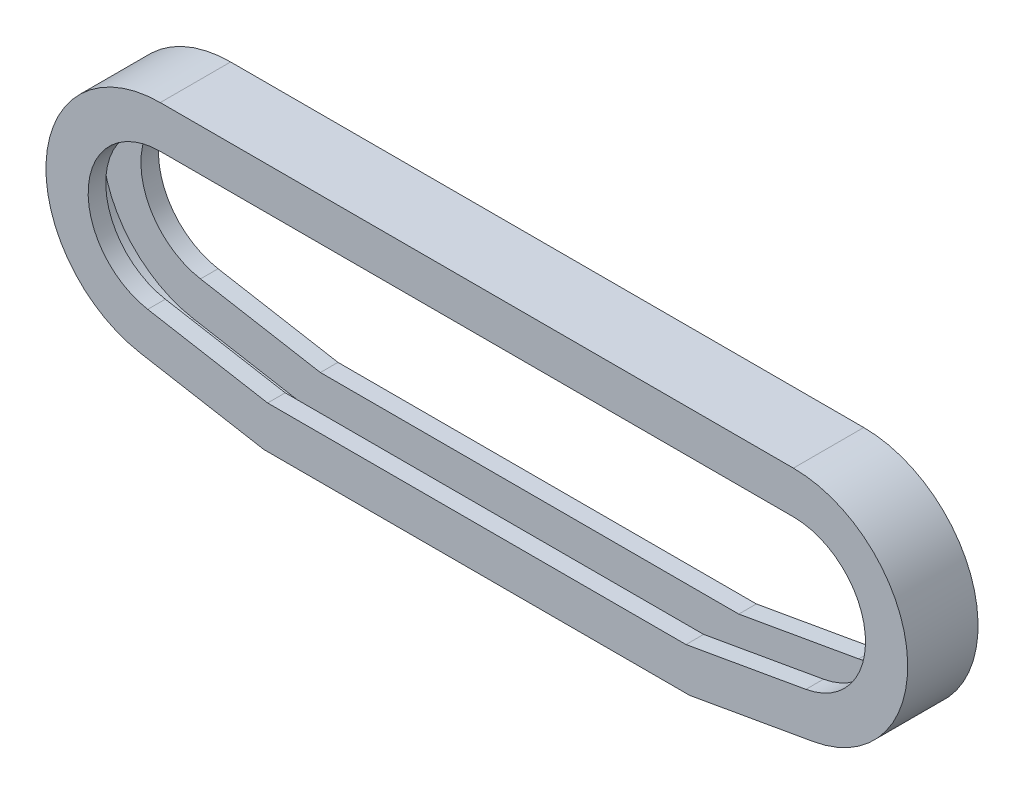
SolidWorks part; units mm, degrees
ref_plane "Front Plane" through (0, 0, 0) normal (0, 0, 1) x (1, 0, 0)
ref_plane "Top Plane" through (0, 0, 0) normal (0, 1, 0) x (1, 0, 0)
ref_plane "Right Plane" through (0, 0, 0) normal (1, 0, 0) x (0, 0, -1)
sketch "Sketch2" plane through (0, 0, 0) normal (0, 0, 1) x (1, 0, 0)
  line L0 (90, 0) -> (-90, 0) construction
  line L1 (0, 0) -> (0, -32.1986) construction
  line L2 (-60, -32.1986) -> (-94.6017, -26.0974) construction
  line L3 (60, -32.1986) -> (94.6017, -26.0974) construction
  line L4 (-90, 26.5) -> (90, 26.5) construction
  line L5 (-60, -32.1986) -> (60, -32.1986) construction
  line L6 (-90, 0) -> (-94.6017, -26.0974) construction
  line L7 (-90, 32.5) -> (90, 32.5)
  line L8 (60.5249, -38.1986) -> (95.6436, -32.0063)
  line L9 (-60.5249, -38.1986) -> (60.5249, -38.1986)
  line L10 (-60.5249, -38.1986) -> (-95.6436, -32.0063)
  line L11 (-90, 20.5) -> (90, 20.5)
  line L12 (59.4751, -26.1986) -> (93.5598, -20.1886)
  line L13 (-59.4751, -26.1986) -> (59.4751, -26.1986)
  line L14 (-59.4751, -26.1986) -> (-93.5598, -20.1886)
  arc A0 (-90, 26.5) -> (-94.6017, -26.0974) centre (-90, 0) ccw construction
  arc A1 (90, 26.5) -> (94.6017, -26.0974) centre (90, 0) cw construction
  arc A2 (90, 32.5) -> (95.6436, -32.0063) centre (90, 0) cw
  arc A3 (-90, 32.5) -> (-95.6436, -32.0063) centre (-90, 0) ccw
  arc A4 (90, 20.5) -> (93.5598, -20.1886) centre (90, 0) cw
  arc A5 (-90, 20.5) -> (-93.5598, -20.1886) centre (-90, 0) ccw
  point P6 (0, 0)
  dimension "D1" = 53
  dimension "D7" = 32.5
  dimension "D8" = 20.5
  dimension "D2" = 180
  dimension "D3" = 30
  dimension "D4" = 100
  dimension "D5" = 6
  dimension "D6" = 6
extrude "Boss-Extrude1" add sketch "Sketch2" along normal mid plane 20
sketch "Sketch8" plane through (0, 0, 0) normal (0, 0, 1) x (1, 0, 0)
  line L18 (60.4374, -37.1986) -> (95.4699, -31.0214)
  line L19 (-60.4374, -37.1986) -> (60.4374, -37.1986)
  line L20 (-95.4699, -31.0214) -> (-60.4374, -37.1986)
  line L21 (90, 31.5) -> (-90, 31.5)
  line L22 (60.4374, -37.1986) -> (95.4699, -31.0214)
  line L23 (-60.4374, -37.1986) -> (60.4374, -37.1986)
  line L24 (-95.4699, -31.0214) -> (-60.4374, -37.1986)
  line L25 (90, 31.5) -> (-90, 31.5)
  arc A12 (95.4699, -31.0214) -> (90, 31.5) centre (90, 0) ccw
  arc A13 (-90, 31.5) -> (-95.4699, -31.0214) centre (-90, 0) ccw
  arc A14 (95.4699, -31.0214) -> (90, 31.5) centre (90, 0) ccw
  arc A15 (-90, 31.5) -> (-95.4699, -31.0214) centre (-90, 0) ccw
  dimension "D1" = 1
extrude "Cut-Extrude1" cut sketch "Sketch8" against normal mid plane 10
